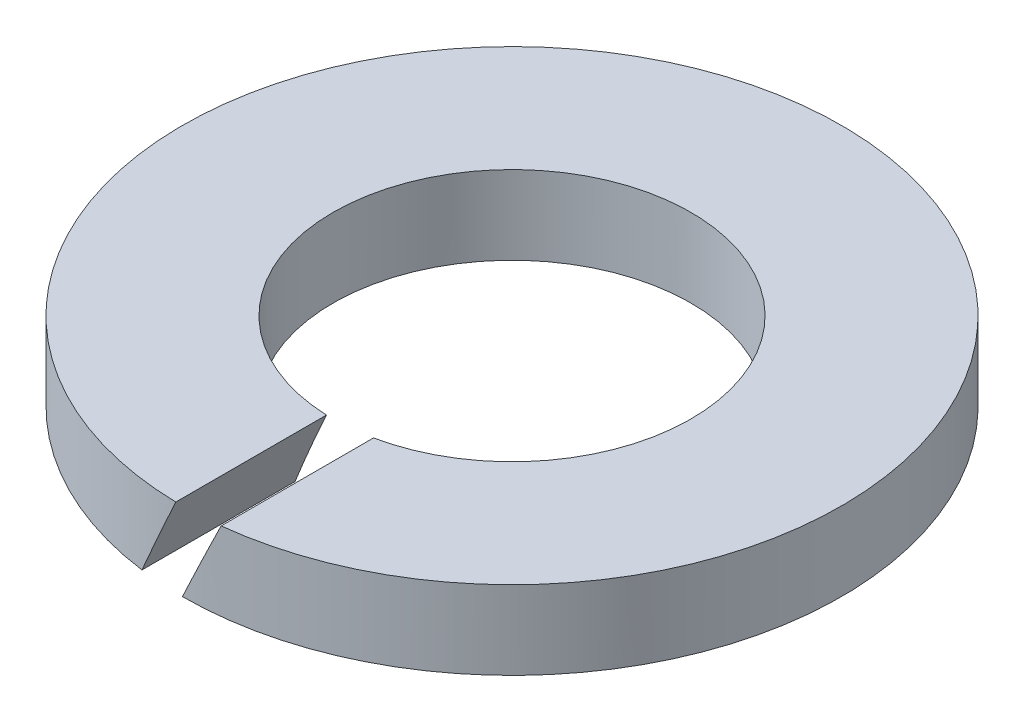
from build123d import *

# Parameters (mm, degrees)
SKETCH_1_R          = 3.775
SKETCH_1_R_2        = 2.05
EXTRUDE_1_DEPTH     = 0.9
CUT_EXTRUDE_1_DEPTH = 6.413986516


with BuildPart() as part:
    # 草图1 → 凸台-拉伸1 (new body)
    with BuildSketch(Plane(origin=(0, 0, 0), x_dir=(1, 0, 0), z_dir=(0, 1, 0))):
        with Locations(Location((0, 0, 0), (0, 0, 270))):
            Circle(SKETCH_1_R)
        with Locations(Location((0, 0, 0), (0, 0, 270))):
            Circle(SKETCH_1_R_2, mode=Mode.SUBTRACT)
    extrude(amount=EXTRUDE_1_DEPTH)

    # 草图2 → 切除-拉伸1 (cut, through all)
    with BuildSketch(Plane.XY):
        Polygon((0, 0), (0.419676892, 0.9), (-0.076843171, 0.9), (-0.496520064, 0), align=None)
    extrude(amount=CUT_EXTRUDE_1_DEPTH, mode=Mode.SUBTRACT)


solid = part.part
